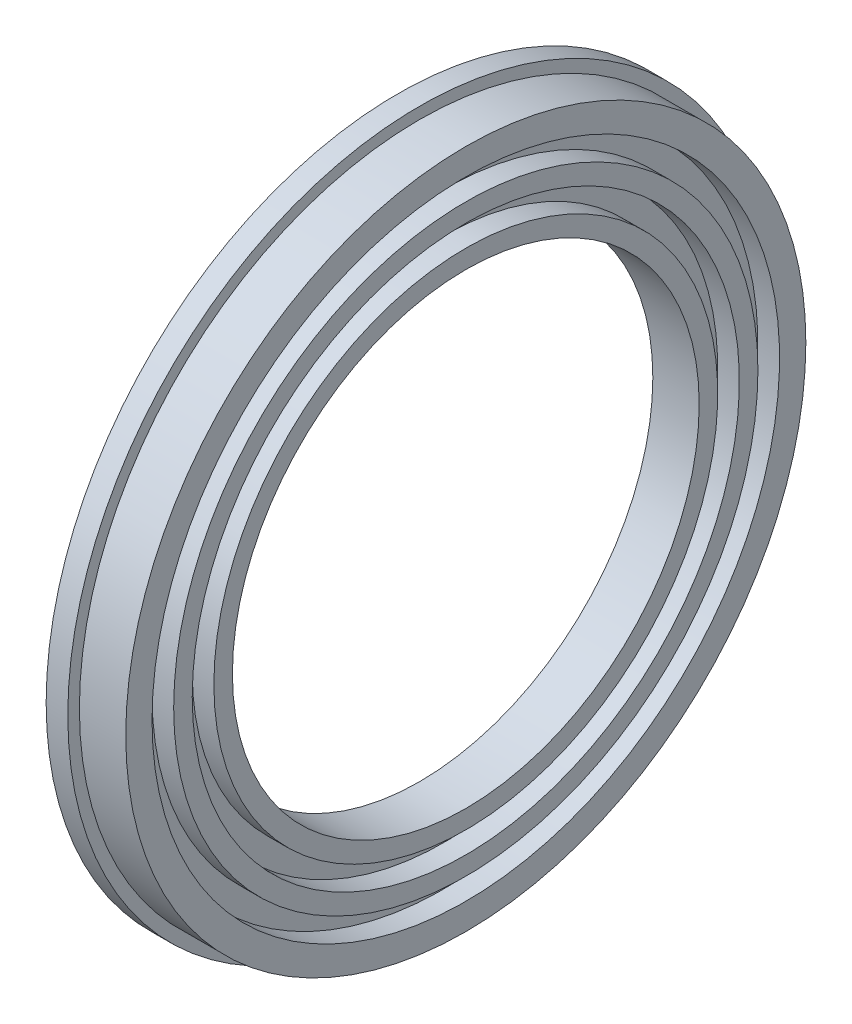
from build123d import *

# Parameters (mm, degrees)
FILLET1_R = 10


with BuildPart() as part:
    # Sketch1 → Revolve1 (revolve)
    with BuildSketch(Plane(origin=(0, 0, 0), x_dir=(1, 0, 0), z_dir=(0, 1, 0)), mode=Mode.PRIVATE) as revolve1_sk:
        Polygon((0, 200), (0, 227.5), (14, 227.5), (14, 220), (44, 220), (44, 203), (30, 203), (30, 189), (44, 189), (44, 177), (30, 177), (30, 163), (44, 163), (44, 151), (14, 151), (14, 200), align=None)
    revolve(revolve1_sk.sketch.rotate(Axis((0, 0, 0), (1, 0, 0)), 180), axis=Axis((0, 0, 0), (1, 0, 0)))

    # Fillet1
    fillet1_edges = [part.edges().sort_by_distance(p)[0] for p in [
        (14, 0, -200),
    ]]
    fillet(fillet1_edges, radius=FILLET1_R)


solid = part.part
